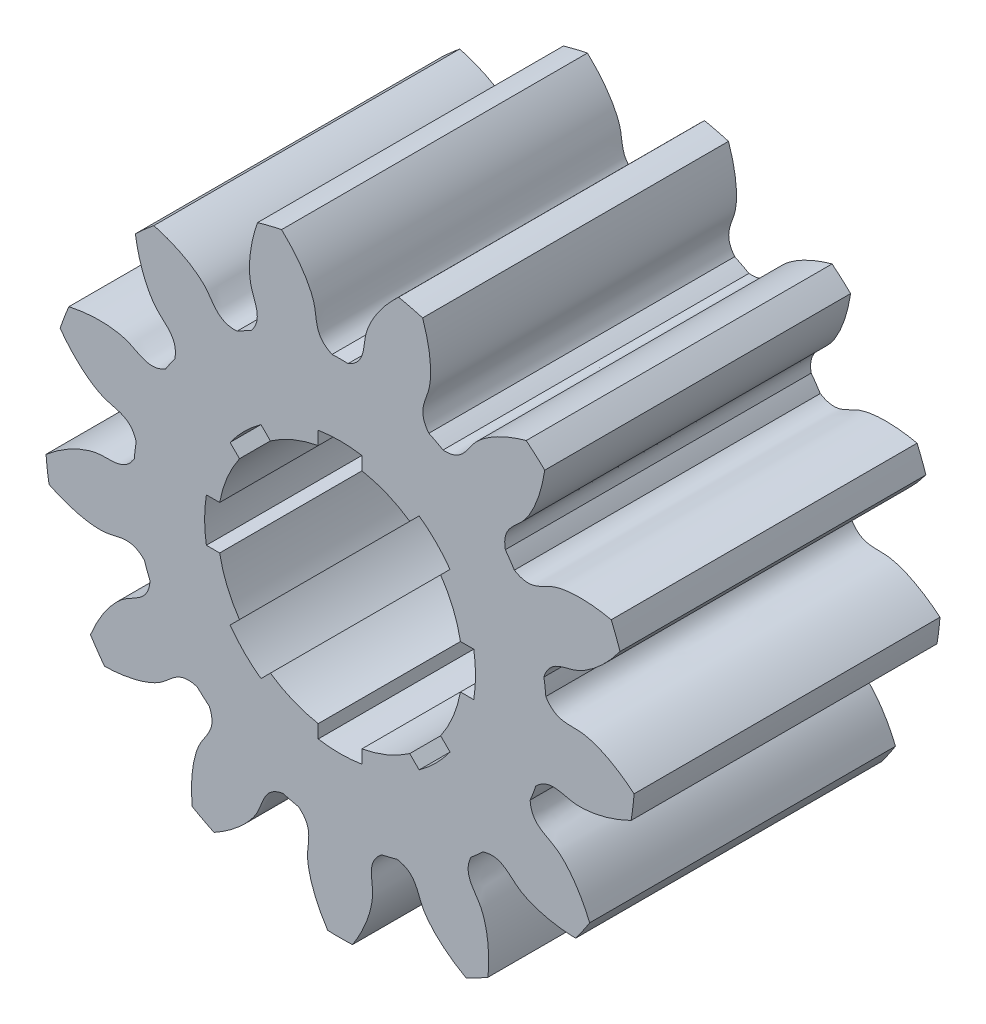
from build123d import *

# Parameters (mm, degrees)
SKETCH_1_R               = 67.5
EXTRUDE_1_DEPTH          = 70
CUT_EXTRUDE_1_DEPTH      = 119.374406018
PATTERN_CIRCULAR_1_COUNT = 13
CUT_EXTRUDE_2_DEPTH      = 119.254967154


with BuildPart() as part:
    # 草图1 → 凸台-拉伸1 (new body)
    with BuildSketch(Plane.XY):
        Circle(SKETCH_1_R)
    extrude(amount=EXTRUDE_1_DEPTH)

    # 草图2 → 切除-拉伸1 (cut, through all)
    with BuildSketch(Plane.XY):
        with BuildLine():
            ThreePointArc((1.829268257, 47.214576961), (0, 47.25), (-1.829268257, 47.214576961))
            add(Edge.make_bspline(
                [(-1.829268257, 47.214576961), (-5.964243007, 49.046283217), (-5.160295599, 52.480391005), (-6.029170045, 55.536484014), (-6.090243946, 55.736259611), (-6.162154184, 55.955670608), (-6.245688331, 56.194359142), (-6.341649308, 56.451938508), (-6.450821195, 56.727999276), (-6.573978901, 57.022107782), (-6.711884387, 57.333806971), (-6.865286986, 57.662616557), (-7.034922495, 58.008033406), (-7.221512645, 58.369531866), (-7.425764476, 58.746564145), (-7.648369743, 59.138560681), (-7.890004332, 59.544930545), (-8.151327682, 59.965061848), (-8.432982221, 60.398322165), (-8.735592806, 60.844058974), (-9.059766183, 61.301600111), (-9.406090448, 61.770254231), (-9.775134532, 62.249311294), (-10.167447681, 62.738043055), (-10.583558966, 63.23570357), (-11.023976792, 63.741529714), (-11.489188426, 64.254741714), (-11.979659538, 64.77454369), (-12.495833752, 65.300124209), (-13.038132215, 65.830656855), (-13.606953173, 66.365300799), (-14.202671572, 66.903201395), (-14.825638663, 67.44349077), (-15.476181626, 67.985288441), (-16.154603209, 68.527701923), (-16.861181382, 69.069827366), (-17.596169006, 69.610750183), (-18.359793518, 70.149545702), (-19.152256631, 70.685279812), (-19.973734049, 71.217009632), (-20.824375204, 71.743784173), (-21.704302999, 72.264645015), (-22.61361358, 72.778626994), (-23.552376113, 73.284758884), (-24.52063258, 73.782064098), (-25.518397636, 74.26956138), (-26.545658262, 74.746265535), (-27.968031612, 75.372065994), (-29.058892742, 75.81309599), (-29.798458362, 76.095343236)],
                knots=[0, 0, 0, 0, 0.219123219, 0.223606469, 0.228617161, 0.234155295, 0.240220869, 0.246813885, 0.253934342, 0.26158224, 0.26975758, 0.27846036, 0.287690582, 0.297448246, 0.30773335, 0.318545896, 0.329885883, 0.341753311, 0.354148181, 0.367070492, 0.380520244, 0.394497437, 0.409002072, 0.424034148, 0.439593665, 0.455680623, 0.472295023, 0.489436863, 0.507106146, 0.525302869, 0.544027034, 0.563278639, 0.583057687, 0.603364175, 0.624198105, 0.645559476, 0.667448288, 0.689864541, 0.712808236, 0.736279372, 0.760277949, 0.784803967, 0.809857427, 0.835438328, 0.86154667, 0.888182454, 0.915345678, 0.943036344, 1, 1, 1, 1], degree=3))
            ThreePointArc((-29.798458362, 76.095343236), (0, 81.721780346), (29.798458362, 76.095343236))
            add(Edge.make_bspline(
                [(1.829268257, 47.214576961), (5.964243007, 49.046283217), (5.160295599, 52.480391005), (6.029170045, 55.536484014), (6.090243946, 55.736259611), (6.162154184, 55.955670608), (6.245688331, 56.194359142), (6.341649308, 56.451938508), (6.450821195, 56.727999276), (6.573978901, 57.022107782), (6.711884387, 57.333806971), (6.865286986, 57.662616557), (7.034922495, 58.008033406), (7.221512645, 58.369531866), (7.425764476, 58.746564145), (7.648369743, 59.138560681), (7.890004332, 59.544930545), (8.151327682, 59.965061848), (8.432982221, 60.398322165), (8.735592806, 60.844058974), (9.059766183, 61.301600111), (9.406090448, 61.770254231), (9.775134532, 62.249311294), (10.167447681, 62.738043055), (10.583558966, 63.23570357), (11.023976792, 63.741529714), (11.489188426, 64.254741714), (11.979659538, 64.77454369), (12.495833752, 65.300124209), (13.038132215, 65.830656855), (13.606953173, 66.365300799), (14.202671572, 66.903201395), (14.825638663, 67.44349077), (15.476181626, 67.985288441), (16.154603209, 68.527701923), (16.861181382, 69.069827366), (17.596169006, 69.610750183), (18.359793518, 70.149545702), (19.152256631, 70.685279812), (19.973734049, 71.217009632), (20.824375204, 71.743784173), (21.704302999, 72.264645015), (22.61361358, 72.778626994), (23.552376113, 73.284758884), (24.52063258, 73.782064098), (25.518397636, 74.26956138), (26.545658262, 74.746265535), (27.968031612, 75.372065994), (29.058892742, 75.81309599), (29.798458362, 76.095343236)],
                knots=[0, 0, 0, 0, 0.219123219, 0.223606469, 0.228617161, 0.234155295, 0.240220869, 0.246813885, 0.253934342, 0.26158224, 0.26975758, 0.27846036, 0.287690582, 0.297448246, 0.30773335, 0.318545896, 0.329885883, 0.341753311, 0.354148181, 0.367070492, 0.380520244, 0.394497437, 0.409002072, 0.424034148, 0.439593665, 0.455680623, 0.472295023, 0.489436863, 0.507106146, 0.525302869, 0.544027034, 0.563278639, 0.583057687, 0.603364175, 0.624198105, 0.645559476, 0.667448288, 0.689864541, 0.712808236, 0.736279372, 0.760277949, 0.784803967, 0.809857427, 0.835438328, 0.86154667, 0.888182454, 0.915345678, 0.943036344, 1, 1, 1, 1], degree=3))
        make_face()
    cut_extrude_1 = extrude(amount=CUT_EXTRUDE_1_DEPTH, mode=Mode.SUBTRACT)

    # 阵列(圆周)1: 切除-拉伸1 ×13 about axis
    pattern_circular_1_axis = Axis((0, 0, 70), (0, 0, -1))
    for i in range(1, PATTERN_CIRCULAR_1_COUNT):
        add(cut_extrude_1.rotate(pattern_circular_1_axis, i * 360 / PATTERN_CIRCULAR_1_COUNT), mode=Mode.SUBTRACT)

    # 草图4 → 切除-拉伸2 (cut, through all)
    with BuildSketch(Plane.XY.offset(70)):
        with BuildLine():
            Line((-5, 30.594117082), (-5, 27.549954628))
            ThreePointArc((-5, 27.549954628), (-10.715136106, 25.86862691), (-15.945225833, 23.016293645))
            Line((-15.945225833, 23.016293645), (-18.097773747, 25.168841559))
            ThreePointArc((-18.097773747, 25.168841559), (-21.920310217, 21.920310217), (-25.168841559, 18.097773747))
            Line((-25.168841559, 18.097773747), (-23.016293645, 15.945225833))
            ThreePointArc((-23.016293645, 15.945225833), (-25.86862691, 10.715136106), (-27.549954628, 5))
            Line((-27.549954628, 5), (-30.594117082, 5))
            ThreePointArc((-30.594117082, 5), (-31, 0), (-30.594117082, -5))
            Line((-30.594117082, -5), (-27.549954628, -5))
            ThreePointArc((-27.549954628, -5), (-25.86862691, -10.715136106), (-23.016293645, -15.945225833))
            Line((-23.016293645, -15.945225833), (-25.168841559, -18.097773747))
            ThreePointArc((-25.168841559, -18.097773747), (-21.920310217, -21.920310217), (-18.097773747, -25.168841559))
            Line((-18.097773747, -25.168841559), (-15.945225833, -23.016293645))
            ThreePointArc((-15.945225833, -23.016293645), (-10.715136106, -25.86862691), (-5, -27.549954628))
            Line((-5, -27.549954628), (-5, -30.594117082))
            ThreePointArc((-5, -30.594117082), (0, -31), (5, -30.594117082))
            Line((5, -30.594117082), (5, -27.549954628))
            ThreePointArc((5, -27.549954628), (10.715136106, -25.86862691), (15.945225833, -23.016293645))
            Line((15.945225833, -23.016293645), (18.097773747, -25.168841559))
            ThreePointArc((18.097773747, -25.168841559), (21.920310217, -21.920310217), (25.168841559, -18.097773747))
            Line((25.168841559, -18.097773747), (23.016293645, -15.945225833))
            ThreePointArc((23.016293645, -15.945225833), (25.86862691, -10.715136106), (27.549954628, -5))
            Line((27.549954628, -5), (30.594117082, -5))
            ThreePointArc((30.594117082, -5), (31, 0), (30.594117082, 5))
            Line((30.594117082, 5), (27.549954628, 5))
            ThreePointArc((27.549954628, 5), (25.86862691, 10.715136106), (23.016293645, 15.945225833))
            Line((23.016293645, 15.945225833), (25.168841559, 18.097773747))
            ThreePointArc((25.168841559, 18.097773747), (21.920310217, 21.920310217), (18.097773747, 25.168841559))
            Line((18.097773747, 25.168841559), (15.945225833, 23.016293645))
            ThreePointArc((15.945225833, 23.016293645), (10.715136106, 25.86862691), (5, 27.549954628))
            Line((5, 27.549954628), (5, 30.594117082))
            ThreePointArc((5, 30.594117082), (0, 31), (-5, 30.594117082))
        make_face()
    extrude(amount=-CUT_EXTRUDE_2_DEPTH, mode=Mode.SUBTRACT)


solid = part.part
